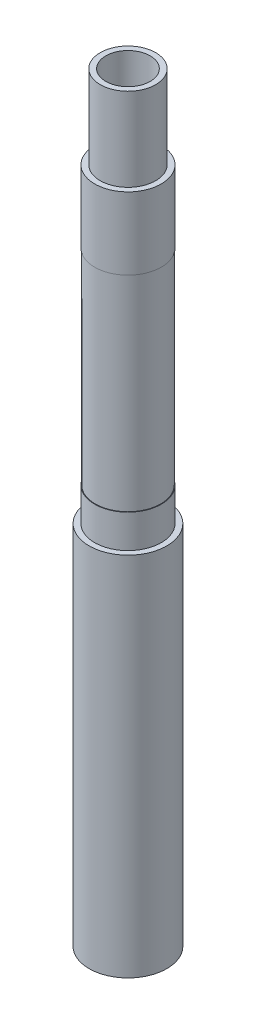
from build123d import *

# Parameters (mm, degrees)
CUT_EXTRUDE1_REACH = 688.786
SKETCH2_R          = 20


with BuildPart() as part:
    # Sketch1 → Revolve1 (revolve)
    with BuildSketch(Plane.XY, mode=Mode.PRIVATE) as revolve1_sk:
        Polygon((0, 0), (35, 0), (35, 330), (30, 330), (30, 360), (29.5, 360), (29.5, 545), (30, 545), (30, 610), (25, 610), (25, 685), (0, 685), align=None)
    revolve(revolve1_sk.sketch.rotate(Axis((0, 685, 0), (0, -1, 0)), 180), axis=Axis((0, 685, 0), (0, -1, 0)))

    # Sketch2 → Cut-Extrude1 (cut, up to next)
    with BuildSketch(Plane(origin=(0, 685, 0), x_dir=(1, 0, 0), z_dir=(0, 1, 0)), mode=Mode.PRIVATE) as cut_extrude1_sk1:
        with Locations(Location((0, 0, 0), (0, 0, 180))):
            Circle(SKETCH2_R)
    cut_extrude1_tool1 = extrude(cut_extrude1_sk1.sketch, amount=-CUT_EXTRUDE1_REACH, mode=Mode.PRIVATE) & part.part
    add(cut_extrude1_tool1.solids().sort_by_distance((0, 685, 0))[0], mode=Mode.SUBTRACT)


solid = part.part
